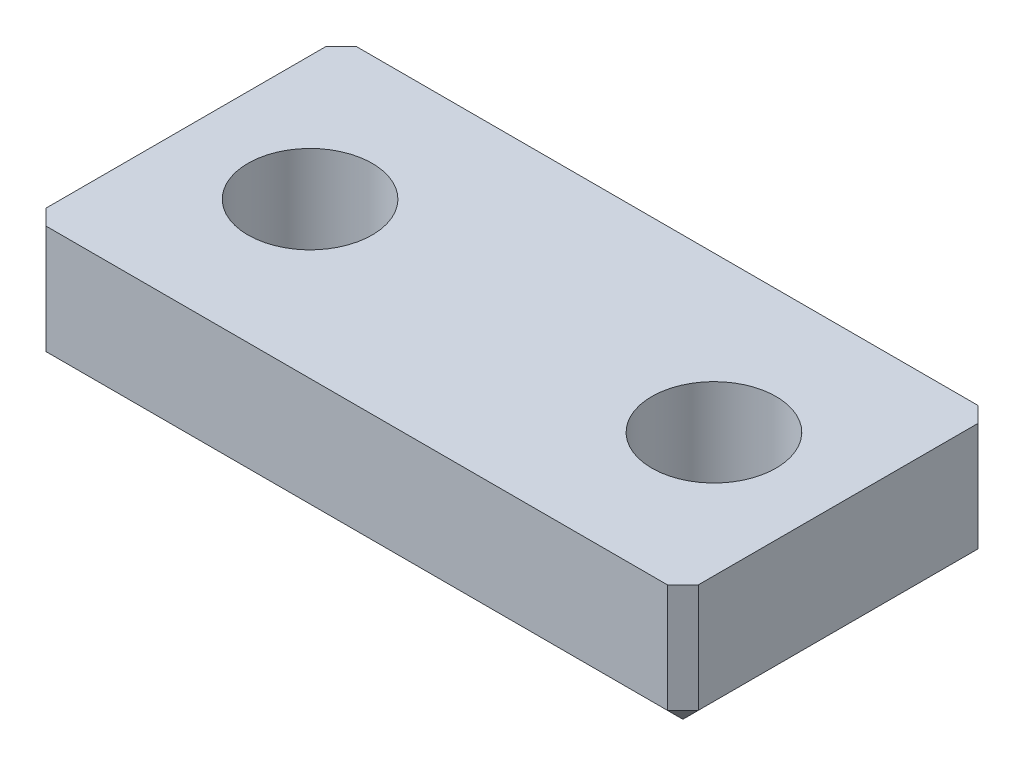
from build123d import *

# Parameters (mm, degrees)
SKETCH1_W           = 21
SKETCH1_H           = 4
BOSS_EXTRUDE1_DEPTH = 10
SKETCH2_R           = 2
CUT_EXTRUDE1_DEPTH  = 10
CHAMFER2_SIZE       = 0.5


with BuildPart() as part:
    # Sketch1 → Boss-Extrude1 (new body)
    with BuildSketch(Plane.XY):
        with Locations((10.5, -2)):
            Rectangle(SKETCH1_W, SKETCH1_H)
    extrude(amount=BOSS_EXTRUDE1_DEPTH)

    # Sketch2 → Cut-Extrude1 (cut)
    with BuildSketch(Plane(origin=(0, 0, 0), x_dir=(1, 0, 0), z_dir=(0, 1, 0))):
        with Locations(Location((17, -5, 0), (0, 0, 270))):
            Circle(SKETCH2_R)
        with Locations(Location((4, -5, 0), (0, 0, 270))):
            Circle(SKETCH2_R)
    extrude(amount=-CUT_EXTRUDE1_DEPTH, mode=Mode.SUBTRACT)

    # Chamfer2
    chamfer2_edges = [part.edges().sort_by_distance(p)[0] for p in [
        (21, -2, 10),
        (0, -2, 10),
        (21, -2, 0),
        (10.5, -4, 0),
        (0, -2, 0),
        (10.5, -4, 10),
        (21, -4, 5),
        (0, -4, 5),
    ]]
    chamfer(chamfer2_edges, length=CHAMFER2_SIZE)


solid = part.part
